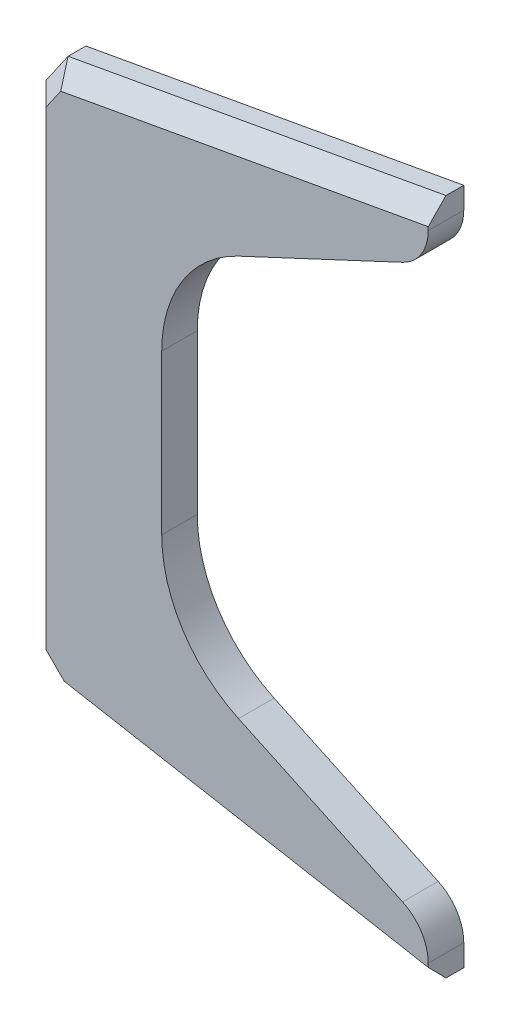
SolidWorks part; units mm, degrees
ref_plane "Front Plane" through (0, 0, 0) normal (0, 0, 1) x (1, 0, 0)
ref_plane "Top Plane" through (0, 0, 0) normal (0, 1, 0) x (1, 0, 0)
ref_plane "Right Plane" through (0, 0, 0) normal (1, 0, 0) x (0, 0, -1)
sketch "Sketch1" plane through (0, 0, 0) normal (0, 0, 1) x (1, 0, 0)
  line L0 (0, -120) -> (0, 120)
  line L1 (0, 120) -> (180, 152.55)
  line L2 (180, 152.55) -> (180, 142.8641)
  line L3 (168.4682, 124.7454) -> (94.5953, 90.219)
  line L4 (60, 35.8627) -> (60, -35.7627)
  line L5 (94.5953, -90.119) -> (168.4682, -124.6454)
  line L6 (180, -142.7641) -> (180, -152.55)
  line L7 (180, -152.55) -> (0, -120)
  line L8 (0, 0) -> (81.9386, 0) construction
  arc A0 (180, -142.7641) -> (168.4682, -124.6454) centre (160, -142.7641) ccw
  arc A1 (180, 142.8641) -> (168.4682, 124.7454) centre (160, 142.8641) cw
  arc A2 (94.5953, -90.119) -> (60, -35.7627) centre (120, -35.7627) cw
  arc A3 (60, 35.8627) -> (94.5953, 90.219) centre (120, 35.8627) cw
  point P17 (60, -73.95)
  point P20 (60, 74.05)
  dimension "D12" = 20
  dimension "D13" = 60
  dimension "D1" = 60
  dimension "D2" = 240
  dimension "D3" = 240
  dimension "D4" = 305.1
  dimension "D5" = 305.1
  dimension "D6" = 180
  dimension "D7" = 180
  dimension "D8" = 148.1
  dimension "D9" = 148
  dimension "D10" = 14.8
  dimension "D11" = 14.8
extrude "Boss-Extrude1" add sketch "Sketch1" along normal blind 16
chamfer "Chamfer1" distance 10 angle 45 2 edges at (0, 120, 8) (0, -120, 8)
chamfer "Chamfer2" distance 8 angle 45 5 edges at (94.9202, 137.1647, 16) (4.9202, 114.687, 16) (6.1038, -116.1038, 16) (96.1038, -137.3788, 16) (0, -1.2028, 16)
